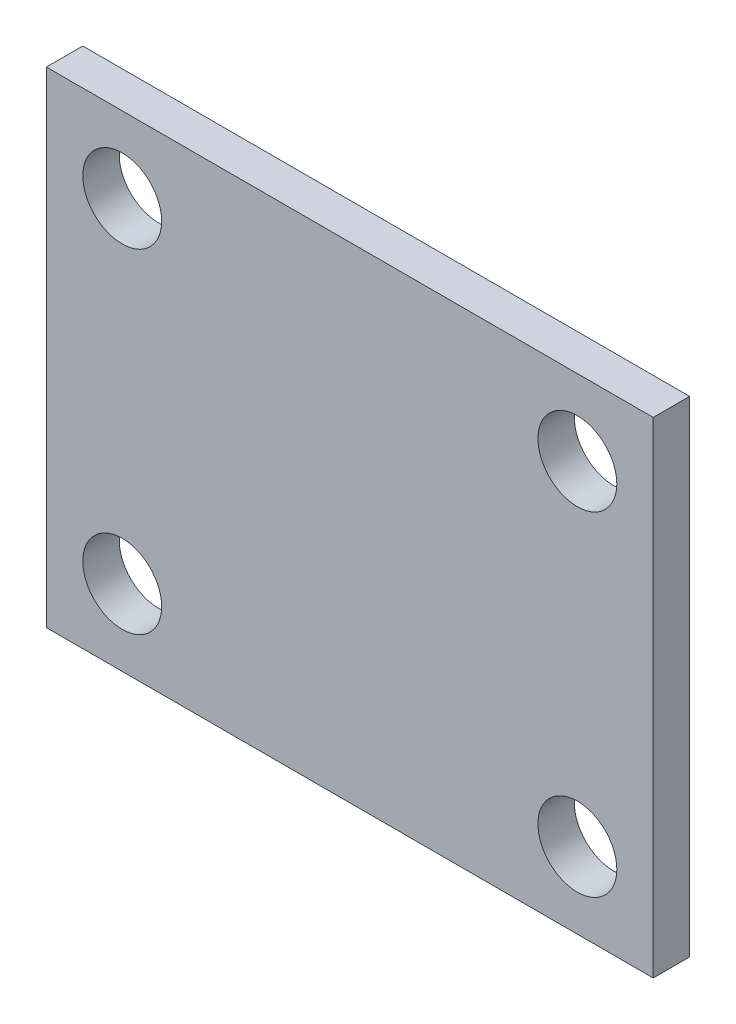
SolidWorks part; units mm, degrees
material "1023 碳钢板 (SS)"
ref_plane "Front Plane" through (0, 0, 0) normal (0, 0, 1) x (1, 0, 0)
ref_plane "Top Plane" through (0, 0, 0) normal (0, 1, 0) x (1, 0, 0)
ref_plane "Right Plane" through (0, 0, 0) normal (1, 0, 0) x (0, 0, -1)
sketch "Sketch1" plane through (0, 0, 0) normal (0, 0, 1) x (1, 0, 0)
  line L1 (50, 40) -> (-50, 40)
  line L2 (50, 40) -> (50, -40)
  line L3 (50, -40) -> (-50, -40)
  line L4 (-50, 40) -> (-50, -40)
  line L5 (50, 40) -> (-50, -40) construction
  line L6 (50, -40) -> (-50, 40) construction
  point P0 (0, 0)
  dimension "D1" = 100
  dimension "D2" = 80
extrude "Boss-Extrude1" add sketch "Sketch1" along normal blind 6
sketch "Sketch2" plane through (0, 0, 6) normal (0, 0, 1) x (1, 0, 0)
  line L1 (37.5, 27.5) -> (-37.5, 27.5) construction
  line L2 (37.5, 27.5) -> (37.5, -27.5) construction
  line L3 (37.5, -27.5) -> (-37.5, -27.5) construction
  line L4 (-37.5, 27.5) -> (-37.5, -27.5) construction
  line L5 (37.5, 27.5) -> (-37.5, -27.5) construction
  line L6 (37.5, -27.5) -> (-37.5, 27.5) construction
  circle A0 centre (-37.5, 27.5) radius 6.5
  circle A1 centre (37.5, 27.5) radius 6.5
  circle A2 centre (37.5, -27.5) radius 6.5
  circle A3 centre (-37.5, -27.5) radius 6.5
  point P0 (0, 0)
  dimension "D3" = 13
  dimension "D1" = 75
  dimension "D2" = 55
extrude "Cut-Extrude1" cut sketch "Sketch2" against normal blind 6
